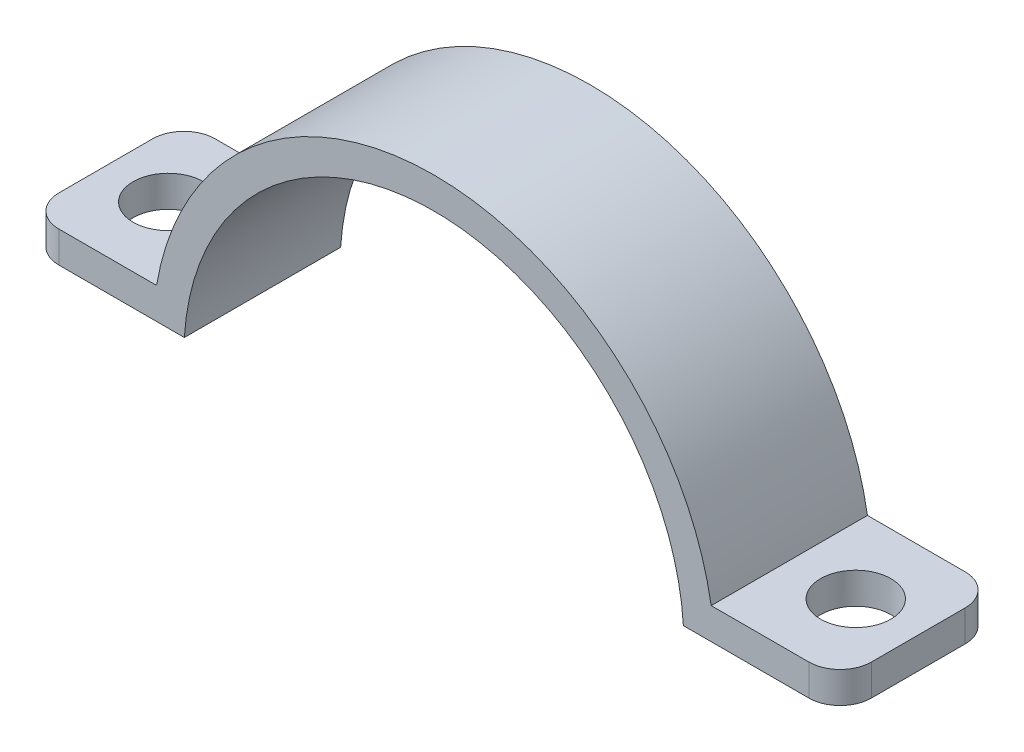
SolidWorks part; units mm, degrees
material "SUS304"
ref_plane "Front Plane" through (0, 0, 0) normal (0, 0, 1) x (1, 0, 0)
ref_plane "Top Plane" through (0, 0, 0) normal (0, 1, 0) x (1, 0, 0)
ref_plane "Right Plane" through (0, 0, 0) normal (1, 0, 0) x (0, 0, -1)
sketch "Sketch1" plane through (0, 0, 0) normal (0, 0, 1) x (1, 0, 0)
  line L0 (0, 0) -> (-10.0313, 0)
  line L1 (31.9374, 0) -> (41.9687, 0)
  arc A0 (0, 0) -> (31.9374, 0) centre (15.9687, -1) cw
  dimension "D1" = 16
  dimension "D3" = 1
  dimension "D2" = 52
extrude "Extrude-Thin1" add sketch "Sketch1" against normal blind 10 thin
hole_wizard "M4 Clearance Hole1" positions "Sketch3" profile "Sketch2" hole size "M4" standard "ISO"
sketch "Sketch3" plane through (0, 2, 0) normal (0, 1, 0) x (1, 0, 0)
  line L0 (-10.0313, 5) -> (41.9687, 5) construction
  line L1 (-10.0313, 10) -> (-10.0313, 0) construction
  line L2 (41.9687, 10) -> (41.9687, 0) construction
  line L3 (15.9687, 5) -> (15.9687, 0) construction
  line L4 (-1.7795, 0) -> (33.717, 0) construction
  point P9 (-6.0313, 5)
  point P11 (37.9687, 5)
  dimension "D1" = 44
sketch "Sketch2" plane through (-6.0313, 2, -5) normal (1, 0, 0) x (0, 0, 1)
  line L0 (0, 0) -> (0, 125.8519)
  line L1 (0, 125.8519) -> (2.25, 124.5)
  line L2 (2.25, 124.5) -> (2.25, 0)
  line L5 (2.25, 0) -> (0, 0)
  line L10 (0, 125.8519) -> (-2.25, 124.5) construction
  line L11 (0, -6.35) -> (0, 107.95) construction
  dimension "孔直径" = 4.5
  dimension "孔深度" = 124.5
  dimension "导头角度" = 118
fillet "Fillet1" radius 2 4 edges at (41.9687, 1, -10) (41.9687, 1, 0) (-10.0313, 1, 0) (-10.0313, 1, -10)
